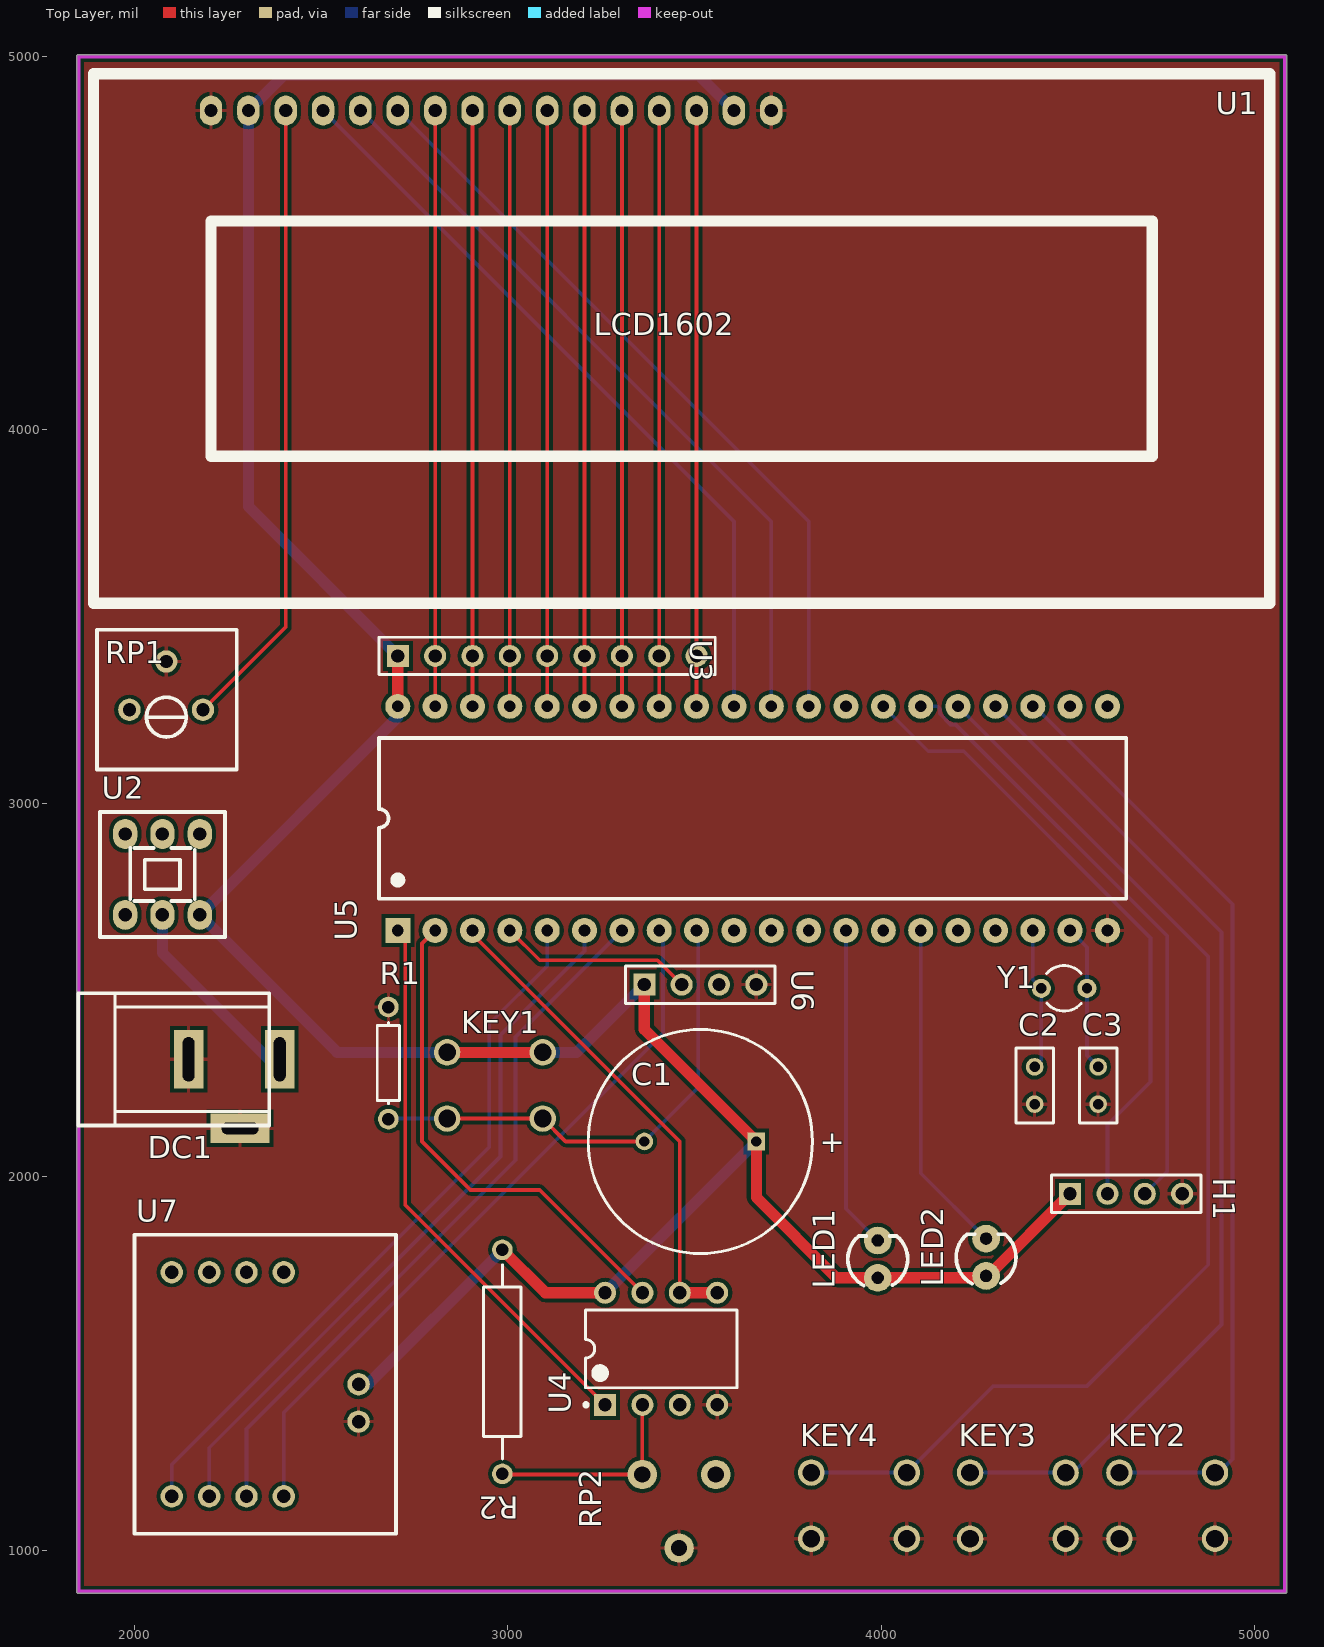
[diagram p0: Top Layer view]
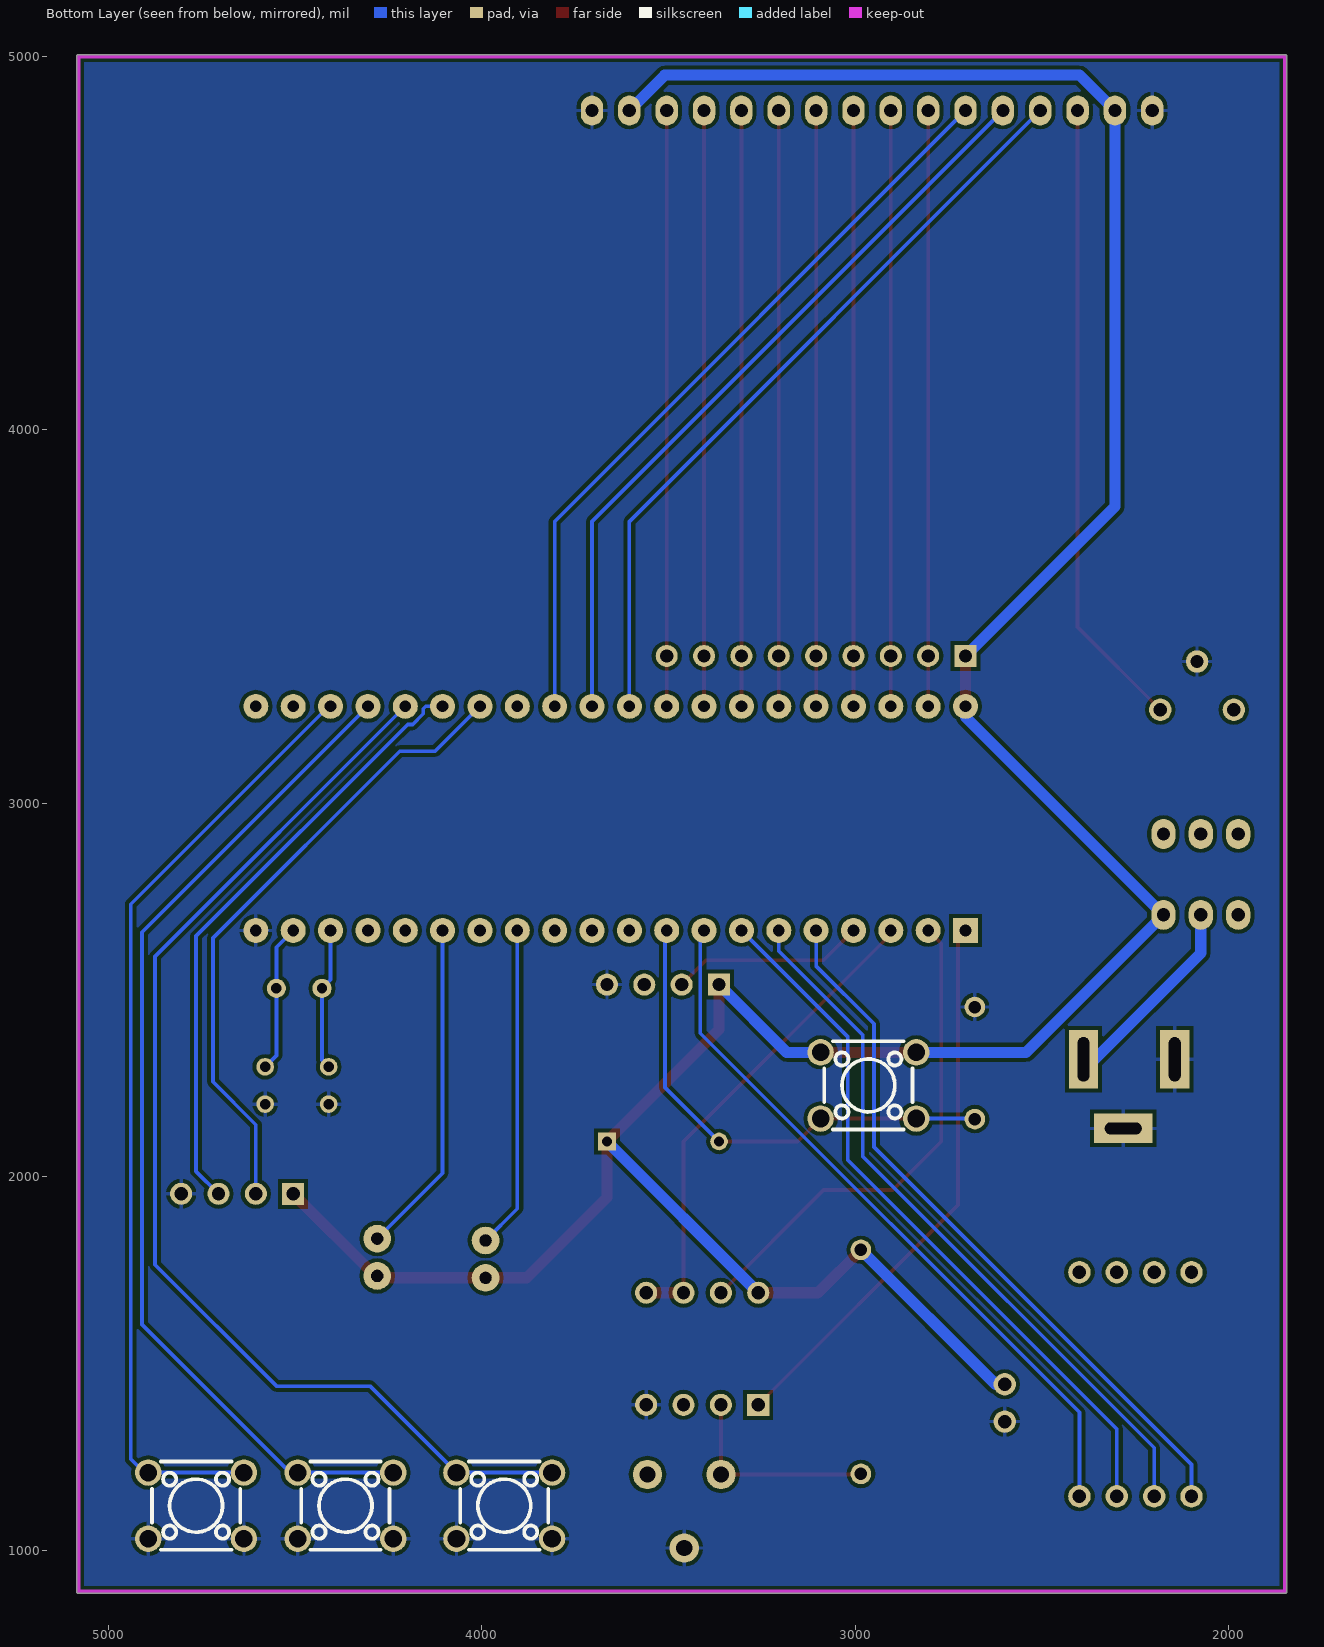
[diagram p1: Bottom Layer view, seen from below]
# Altium PCB MISC80828.PcbDoc
Units mil, origin at the board's own origin, x right, y up, seen from the top; angles counter-clockwise.
Board outline 3240.03 x 4120.03 mil, 2 copper layers (Top Layer, Bottom Layer); 23 components, 34 nets, 138 pads, 0 vias.

## Layer stack, top to bottom (the 12.6 mil dielectric is the usual default, probably not edited)
Top Solder: solder mask 0.4, Solder Resist, Dk 3.5
Top Layer: signal copper 1.4
Dielectric 1: dielectric 12.6, FR-4, Dk 4.8
Bottom Layer: signal copper 1.4
Bottom Solder: solder mask 0.4, Solder Resist, Dk 3.5

## Board outline
1844.98,890 ccw(c1850,890) 1850,884.99 5080,884.99 ccw(c5080,890) 5085.02,890 5085.02,5000 ccw(c5080,5000) 5080,5005.02 1850,5005.02 ccw(c1850,5000) 1844.98,5000

## Design rules (kind name [scope] priority, off if disabled: settings)
Clearance [All] p1: gap=10
MinimumSolderMaskSliver [All] p1: minsoldermaskwidth=0
PolygonConnect [All] p1: connectstyle=Relief reliefconductorwidth=10 reliefentries=4 polygonreliefangle="90 Angle" airgapwidth=10
RoutingVias [All] p1: holewidth=28 width=50 viastyle="Through Hole" minholewidth=28 minwidth=50 maxholewidth=28 maxwidth=50
SilkToSilkClearance [All] p1: silktosilkclearance=0
SilkToSolderMaskClearance [IsPad] p1: minsilkscreentomaskgap=0 clearancetoexposedcopper=TRUE
SolderMaskExpansion [All] p1: expansion=4
Width [All] p1: maxlimit=30 minlimit=10 preferedwidth=10
27 further rules are at their usual default settings.

## Components (designator, comment, footprint, x,y, rotation, side; value= is the part's Value field where it differs from the comment)
C1 "10uF" RB7.6-15 3515,2095 r0 top
C2 "33p" RAD-0.1 4410,2245 r90 top
C3 "33p" RAD-0.1 4580,2245 r90 top
DC1 "DC-005" DC-005 2389.09,2315 r180 top
H1 "Pressure sensor" HDR1X4 4505,1955 r0 top
KEY1 "button6*6*8.5" 四脚轻触开关 2965,2245 r180 top
KEY2 "button6*6*8.5" 四脚轻触开关 4765,1120 r0 top
KEY3 "button6*6*8.5" 四脚轻触开关 4365,1120 r0 top
KEY4 "button6*6*8.5" 四脚轻触开关 3940,1120 r0 top
LED1 "LED-0603_R" LED3MM 3990,1780 r90 top
LED2 "LED-0603_R" LED3MM 4280,1785 r90 top
R1 "10k" AXIAL-0.3 2680,2305 r90 top
R2 "Photoresistor" AXIAL-0.6 2985,1505 r270 top
RP1 "502" 电位器 2087.01,3265.9 r0 top
RP2 "103" RM065 3460,1105 r180 top
U1 "1602" LCD1602 2205,4855 r0 top
U2 "Self-locking switch_power supply" 自锁开关 2075,2810 r0 top
U3 "respack-8" HDR1X9 2705,3395 r0 top
U4 "ADC0832" DIP-8 3410,1540 r90 top
U5 "STC89C52RC" DIP40 3655,2960 r90 top
U6 "DHT11" HDR1X4 3365,2515 r0 top
U7 "ULN2003 stepper motor driver" ULN2003 2350,1445 r90 top
Y1 "12M" R38 4488.98,2505 r270 top

## Footprints (in the part's own frame and the unit in brackets; to place one, negate y for a bottom-side part, rotate by r counter-clockwise, add the part's x,y. Pads: shape width x height; smd on the part's side, far side on the other; paste and mask are expansions set on the pad)
AXIAL-0.3 [mm] "Axial Device, Thru-Hole; 2 Leads; 0.3 in Pin Spacing"
  round 1.4 hole 0.85: 1(-3.81,0) 2(3.81,0)
  silkscreen extent -2.77,-0.76 2.77,0.76
AXIAL-0.6 [mm] "Axial Device, Thru-Hole; 2 Leads; 0.6 in Pin Spacing"
  round 1.4 hole 0.85: 1(-7.62,0) 2(7.62,0)
  silkscreen extent -6.6,-1.27 6.6,1.27
DC-005 [mm] "5.5X2.1mm"
  rect 2x4 hole 0.8 slot 3 at 90 deg: 1(0,0) 2(6.2,0)
  rect 4x2 hole 0.8 slot 2.5 at 0 deg: 3(2.7,4.7)
  silkscreen extent 0.72,-4.5 13.7,4.5, body extent -0.4,-4.52 13.65,4.78, height 11.2
DIP40 [mm]
  rect 1.7x1.7 hole 0.8: 1(-7.62,24.13)
  round 1.7 hole 0.8: 2(-7.62,21.59) 3(-7.62,19.05) 4(-7.62,16.51) 5(-7.62,13.97) 6(-7.62,11.43) 7(-7.62,8.89) 8(-7.62,6.35) 9(-7.62,3.81) 10(-7.62,1.27) 11(-7.62,-1.27) 12(-7.62,-3.81) 13(-7.62,-6.35) 14(-7.62,-8.89) 15(-7.62,-11.43) 16(-7.62,-13.97) 17(-7.62,-16.51) 18(-7.62,-19.05) 19(-7.62,-21.59) 20(-7.62,-24.13) 21(7.62,-24.13) 22(7.62,-21.59) 23(7.62,-19.05) 24(7.62,-16.51) 25(7.62,-13.97) 26(7.62,-11.43) 27(7.62,-8.89) 28(7.62,-6.35) 29(7.62,-3.81) 30(7.62,-1.27) 31(7.62,1.27) 32(7.62,3.81) 33(7.62,6.35) 34(7.62,8.89) 35(7.62,11.43) 36(7.62,13.97) 37(7.62,16.51) 38(7.62,19.05) 39(7.62,21.59) 40(7.62,24.13)
  silkscreen extent -5.46,-25.4 5.46,25.4, body extent -7.91,-26.19 7.65,26.16, height 4.7
DIP-8 [mm] "DIP; 8 Leads; Row Spacing 7.62 mm; Pitch 2.54 mm"
  rect 1.5x1.5 hole 0.9: 1(-3.81,3.81)
  round 1.5 hole 0.9: 2(-3.81,1.27) 3(-3.81,-1.27) 4(-3.81,-3.81) 5(3.81,-3.81) 6(3.81,-1.27) 7(3.81,1.27) 8(3.81,3.81)
  silkscreen extent -3.93,-5.15 2.65,5.23, body extent -3.6,-5.15 3.6,5.15, height 5.08
HDR1X4 [mm] "Connector; Header; 4 Position"
  rect 1.5x1.5 hole 0.9: 1(0,0)
  round 1.5 hole 0.9: 2(2.54,0) 3(5.08,0) 4(7.62,0)
  silkscreen extent -1.27,-1.27 8.89,1.27
HDR1X9 [mm] "Connector; Header; 9 Position"
  rect 1.5x1.5 hole 0.9: 1(0,0)
  round 1.5 hole 0.9: 2(2.54,0) 3(5.08,0) 4(7.62,0) 5(10.16,0) 6(12.7,0) 7(15.24,0) 8(17.78,0) 9(20.32,0)
  silkscreen extent -1.27,-1.27 21.59,1.27
LCD1602 [mil]
  oval 60x80 hole 35.43: 1(0,0) 2(100,0) 3(200,0) 4(300,0) 5(400,0) 6(500,0) 7(600,0) 8(700,0) 9(800,0) 10(900,0) 11(1000,0) 12(1100,0) 13(1200,0) 14(1300,0) 15(1400,0) 16(1500,0)
  silkscreen extent -315,-1319 2835,98, body extent -315,-1357 2854,80, height 414
LED3MM [mil]
  round 74 hole 32 slot 32.2 at 0 deg paste+0 mask+2: 1(-50,0) 2(50,0)
  silkscreen extent -71,-80 62,80
R38 [mm] "Crystal, Thru-Hole; 2 Leads; Body 3.1 x 8.2 mm (Dia.xH)"
  round 1.3 hole 0.7: 1(0,1.55) 2(0,-1.55)
  silkscreen extent -1.55,-1.19 1.55,1.17
RAD-0.1 [mm] "Radial Cap, Thru-Hole; 2 Leads; 0.1 in Pin Spacing"
  round 1.2 hole 0.7: 1(-1.27,0) 2(1.27,0)
  silkscreen extent -2.54,-1.27 2.54,1.27
RB7.6-15 [mm] "Polarized Capacitor (Radial); 2 Leads"
  rect 1.2x1.2 hole 0.7: 1(3.81,0)
  round 1.2 hole 0.7: 2(-3.81,0)
  silkscreen extent -7.62,-7.62 7.62,7.62
RM065 [mm]
  round 2 hole 1.1 paste+0 mask+0.051: 1(-2.449,-2.501) 2(0.05,2.499) 3(2.549,-2.499)
ULN2003 [mil]
  round 60 hole 36 paste+4 mask+4: 1(-300,250) 2(-300,150) 3(-300,50) 4(-300,-50) 5(-100,-250) 6(0,-250) 7(300,250) 8(300,150) 9(300,50) 10(300,-50)
  silkscreen extent -400,-350 400,350
四脚轻触开关 [mm]
  round 1.8 hole 1.2 paste+0 mask+0.102: 1(3.25,2.25) 2(-3.25,2.25) 3(3.25,-2.25) 4(-3.25,-2.25)
电位器 [mil]
  round 60 hole 35.43 paste+0 mask+2: 1(96.41,-15.12) 2(-2.01,114.1) 3(-100.44,-15.12)
  silkscreen extent -187,-175 187,199
自锁开关 [mil]
  oval 65x80 hole 36 paste+0 mask+4: 1(-100,-108.27) 2(0,-108.27) 3(100,-108.27) 4(-100,108.27) 5(0,108.27) 6(100,108.27)
  silkscreen extent -167,-167 167,167

## Part data
H1: library part 气压传感器
R2: library part 光敏
U2: library part 自锁开关_电源供电
U7: library part ULN2003步进电机驱动

## Nets (pads, with @x,y where several pads share a name; then routed paths per layer and width w, separated by ;. In a path a pad name is that pad's centre, name@x,y a point inside that pad or via, vN(x,y) a via of type N, cw(c..) or ccw(c..) an arc to the next point about the centre after c; other vN are vias at no path point)
+5V: C1.1 H1.1 KEY1.3 KEY1.4 LED1.1 LED2.1 R2.1 U1.2 U1.15 U2.3 U3.1 U4.8 U5.40 U6.1 U7.6 | length 8480.9
  Top Layer w30: U5.40 U3.1 ; KEY1.3 KEY1.4 ; R2.1 3100,1690 U4.8 ; U6.1 3365,2395 C1.1 3665,1945 3880,1730 LED1.1 4275,1730 LED2.1 4285,1735 H1.1
  Bottom Layer w30: U7.6 2625,1445 R2.1 ; U5.40 2705,3231.73 U2.3 2543.15,2333.58 KEY1.3 ; U3.1 2305,3795 U1.2 2400,4950 3510,4950 U1.15 ; KEY1.4 3183.58,2333.58 U6.1 ; U4.8 C1.1
GND: C2.1 C3.1 DC1.2 DC1.3 H1.4 KEY2.3 KEY2.4 KEY3.3 KEY3.4 KEY4.3 KEY4.4 R1.2 RP1.2 RP2.2 U1.1 U1.16 U4.4 U5.20 U6.4 U7.5
NetC1_2: C1.2 KEY1.1 KEY1.2 R1.1 U5.9 | length 1340.4
  Top Layer w10: KEY1.1 KEY1.2 3154.37,2095 C1.2
  Bottom Layer w10: R1.1 2681.42,2156.42 KEY1.1 ; C1.2 3509.53,2239.53 3509.53,2660 U5.9
NetC2_2: C2.2 U5.18 Y1.2 | length 381.9
  Bottom Layer w10: U5.18 4405,2527.95 Y1.2 4427.95,2312.95 C2.2
NetC3_2: C3.2 U5.19 Y1.1 | length 396.1
  Bottom Layer w10: U5.19 4550,2615 Y1.1 4550,2325 C3.2
NetDC1_1: DC1.1 U2.2 | length 533.9
  Bottom Layer w30: U2.2 2075,2600 2360,2315 DC1.1
NetH1_2: H1.2 U5.27 | length 1704.4
  Bottom Layer w10: U5.27 4125,3140 4220,3140 4720,2640 4720,2255 4605,2140 H1.2
NetH1_3: H1.3 U5.26 | length 1637.5
  Bottom Layer w10: U5.26 4150,3260 4156.54,3253.46 4156.54,3239.93 4184.93,3211.54 4198.46,3211.54 4765,2645 4765,2015 H1.3
NetKEY2_1: KEY2.1 KEY2.2 U5.23 | length 2557.6
  Bottom Layer w10: U5.23 4410,3260 4940,2730 4940,1245 4903.58,1208.58 KEY2.1 KEY2.2
NetKEY3_1: KEY3.1 KEY3.2 U5.24 | length 2742.8
  Bottom Layer w10: KEY3.2 KEY3.1 4513.58,1208.58 4910,1605 4910,2655 U5.24
NetKEY4_1: KEY4.1 KEY4.2 U5.25 | length 3066
  Bottom Layer w10: KEY4.2 KEY4.1 4299.37,1440 4550,1440 4875,1765 4875,2590 U5.25
NetLED1_2: LED1.2 U5.13 | length 865.2
  Bottom Layer w10: U5.13 3905,1915 LED1.2
NetLED2_2: LED2.2 U5.15 | length 897.5
  Bottom Layer w10: U5.15 4105,2010 LED2.2
NetR2_2: R2.2 RP2.3 U4.2 | length 562
  Top Layer w10: R2.2 2986.6,1203.4 RP2.3 3359.63,1389.63 U4.2
NetRP1_1: RP1.1 U1.3 | length 1696
  Top Layer w10: RP1.1 2405,3472.36 U1.3
NetU1_4: U1.4 U5.31 | length 2050.6
  Bottom Layer w10: U1.4 3605,3755 U5.31
NetU1_5: U1.5 U5.30 | length 2050.6
  Bottom Layer w10: U1.5 3705,3755 U5.30
NetU1_6: U1.6 U5.29 | length 2050.6
  Bottom Layer w10: U1.6 3805,3755 U5.29
NetU1_7: U1.7 U3.2 U5.39 | length 1595
  Top Layer w10: U5.39 U3.2 U1.7
NetU1_8: U1.8 U3.3 U5.38 | length 1595
  Top Layer w10: U5.38 U3.3 U1.8
NetU1_9: U1.9 U3.4 U5.37 | length 1595
  Top Layer w10: U5.37 U3.4 U1.9
NetU1_10: U1.10 U3.5 U5.36 | length 1595
  Top Layer w10: U5.36 U3.5 U1.10
NetU1_11: U1.11 U3.6 U5.35 | length 1595
  Top Layer w10: U5.35 U3.6 U1.11
NetU1_12: U1.12 U3.7 U5.34 | length 1595
  Top Layer w10: U5.34 U3.7 U1.12
NetU1_13: U1.13 U3.8 U5.33 | length 1595
  Top Layer w10: U5.33 U3.8 U1.13
NetU1_14: U1.14 U3.9 U5.32 | length 1595
  Top Layer w10: U5.32 U3.9 U1.14
NetU4_1: U4.1 U5.1 | length 1499.9
  Top Layer w10: U5.1 2725,2640 2725,1925 U4.1
NetU4_5: U4.5 U4.6 U5.3 | length 1299.9
  Top Layer w10: U5.3 2905,2650 3460,2095 U4.6
  Top Layer w30: U4.6 U4.5
NetU4_7: U4.7 U5.2 | length 1337.3
  Top Layer w10: U5.2 2770,2625 2770,2095 2900,1965 3085,1965 U4.7
NetU5_4: U5.4 U6.2 | length 520.1
  Top Layer w10: U5.4 3085,2580 3400,2580 U6.2
NetU5_5: U5.5 U7.1 | length 1931.3
  Bottom Layer w10: U7.1 2100,1230 2950,2080 2950,2410 3105,2565 U5.5
NetU5_6: U5.6 U7.2 | length 1931.3
  Bottom Layer w10: U7.2 2200,1275 2980,2055 2980,2380 3205,2605 U5.6
NetU5_7: U5.7 U7.3 | length 1931.3
  Bottom Layer w10: U7.3 2300,1325 3020,2045 3020,2375 U5.7
NetU5_8: U5.8 U7.4 | length 1939.6
  Bottom Layer w10: U7.4 2400,1370 3415,2385 3415,2650 U5.8
pads on no net: RP1.3 RP2.1 U2.1 U2.4 U2.5 U2.6 U4.3 U5.10 U5.11 U5.12 U5.14 U5.16 U5.17 U5.21 U5.22 U5.28 U6.3 U7.7 U7.8 U7.9 U7.10

## Polygon pours and split planes (outlines as drawn)
GND on Bottom Layer "G" (solid, remove dead copper, pour order 2): 1495,845 5310,845 5190,965 5190,5190 1565,5190 1425,5330
GND on Top Layer "G" (solid, remove dead copper, pour order 4): 1375,5195 1425,5145 5365,5145 5365,720 5245,600 5220,625 1530,625

## Keep-outs
Keep-Out Layer:
  lines w10: 4995,890 5080,890 5080,5000 1850,5000 1850,945 1850,890 5005,890